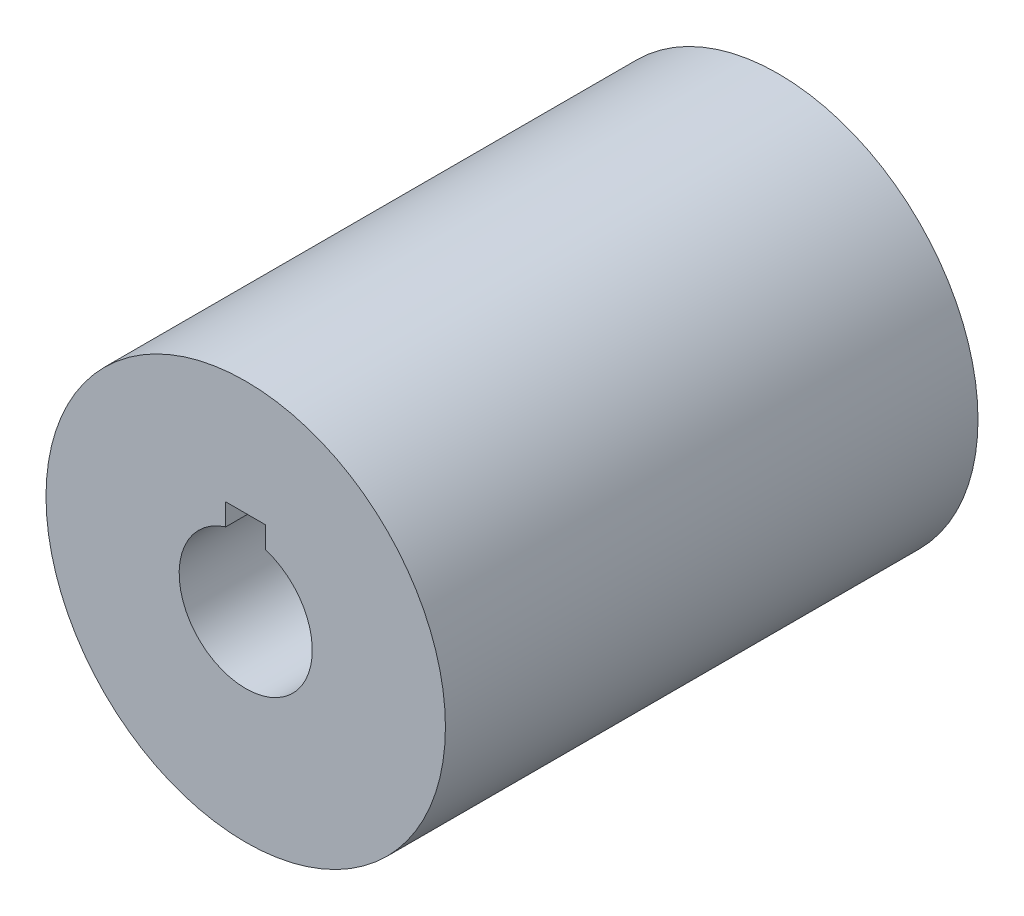
from build123d import *

# Parameters (mm, degrees)
SKETCH1_R           = 30
BOSS_EXTRUDE1_DEPTH = 40
SKETCH2_R           = 10
CUT_EXTRUDE1_DEPTH  = 91.553851381
SKETCH3_R           = 15
CUT_EXTRUDE2_DEPTH  = 40
SKETCH4_W           = 6
SKETCH4_H           = 5.930152299
CUT_EXTRUDE3_DEPTH  = 40
SKETCH5_W           = 6.6
SKETCH5_H           = 8
CUT_EXTRUDE4_DEPTH  = 40


with BuildPart() as part:
    # Sketch1 → Boss-Extrude1 (new, symmetric)
    with BuildSketch(Plane.XY):
        Circle(SKETCH1_R)
    extrude(amount=BOSS_EXTRUDE1_DEPTH, both=True)

    # Sketch2 → Cut-Extrude1 (cut, through all)
    with BuildSketch(Plane.XY.offset(40)):
        Circle(SKETCH2_R)
    extrude(amount=-CUT_EXTRUDE1_DEPTH, mode=Mode.SUBTRACT)

    # Sketch3 → Cut-Extrude2 (cut)
    with BuildSketch(Plane(origin=(0, 0, -40), x_dir=(-1, 0, 0), z_dir=(0, 0, -1))):
        Circle(SKETCH3_R)
    extrude(amount=-CUT_EXTRUDE2_DEPTH, mode=Mode.SUBTRACT)

    # Sketch4 → Cut-Extrude3 (cut)
    with BuildSketch(Plane.XY.offset(40)):
        with Locations((0, 9.834923851)):
            Rectangle(SKETCH4_W, SKETCH4_H)
    extrude(amount=-CUT_EXTRUDE3_DEPTH, mode=Mode.SUBTRACT)

    # Sketch5 → Cut-Extrude4 (cut)
    with BuildSketch(Plane(origin=(0, 0, -40), x_dir=(-1, 0, 0), z_dir=(0, 0, -1))):
        with Locations((15, 0)):
            Rectangle(SKETCH5_W, SKETCH5_H)
    extrude(amount=-CUT_EXTRUDE4_DEPTH, mode=Mode.SUBTRACT)


solid = part.part
